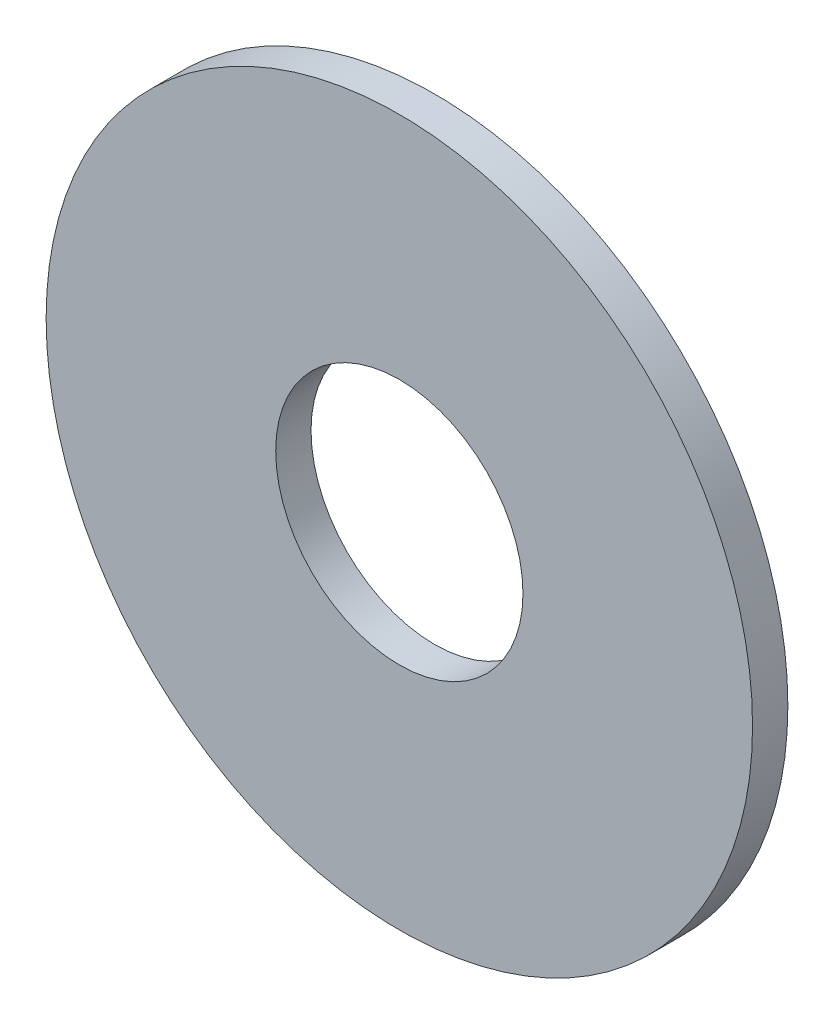
from build123d import *

# Parameters (mm, degrees)
SKETCH1_R           = 10
SKETCH1_R_2         = 3.5
BOSS_EXTRUDE1_DEPTH = 1


with BuildPart() as part:
    # Sketch1 → Boss-Extrude1 (new body)
    with BuildSketch(Plane.XY):
        Circle(SKETCH1_R)
        Circle(SKETCH1_R_2, mode=Mode.SUBTRACT)
    extrude(amount=BOSS_EXTRUDE1_DEPTH)


solid = part.part
